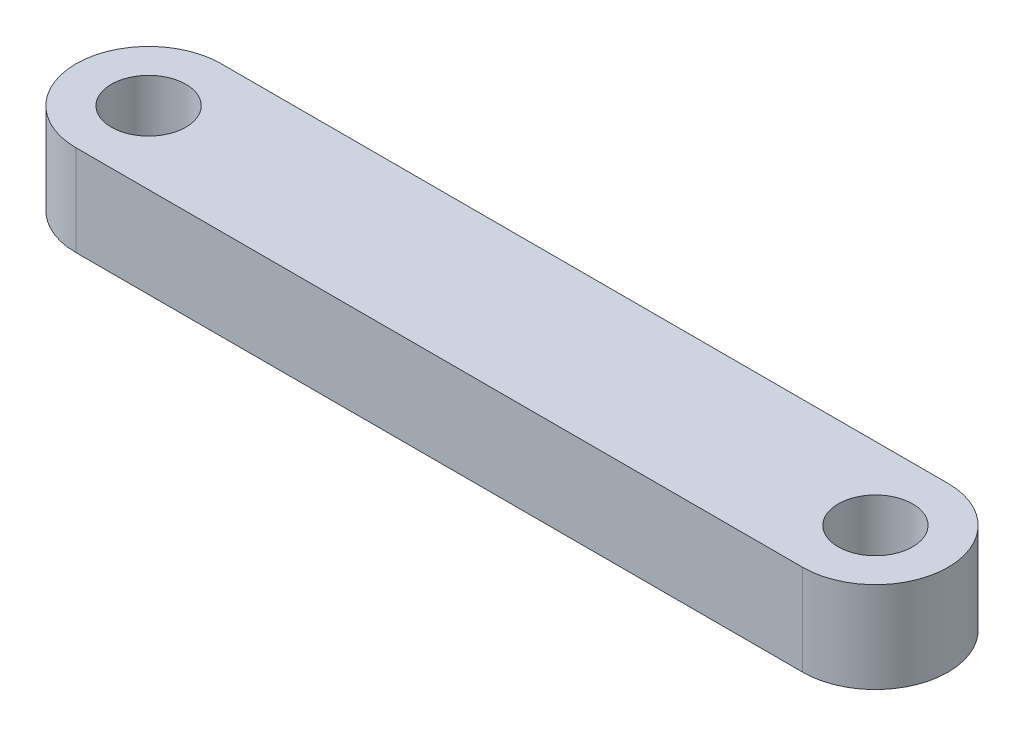
from build123d import *

# Parameters (mm, degrees)
SKETCH1_R           = 2.9
BOSS_EXTRUDE1_DEPTH = 6.35
BOSS_EXTRUDE2_START = -6.35
SKETCH2_R           = 2.9
SKETCH2_R_2         = 2.6035
BOSS_EXTRUDE2_DEPTH = 6.35


with BuildPart() as part:
    # Sketch1 → Boss-Extrude1 (new body)
    with BuildSketch(Plane(origin=(0, 0, 0), x_dir=(1, 0, 0), z_dir=(0, 1, 0))):
        with BuildLine():
            Line((0, 5.08), (50.8, 5.08))
            ThreePointArc((50.8, 5.08), (55.88, 0), (50.8, -5.08))
            Line((50.8, -5.08), (0, -5.08))
            ThreePointArc((0, -5.08), (-5.08, 0), (0, 5.08))
        make_face()
        with Locations(Location((0, 0, 0), (0, 0, 270))):
            Circle(SKETCH1_R, mode=Mode.SUBTRACT)
        with Locations(Location((50.8, 0, 0), (0, 0, 270))):
            Circle(SKETCH1_R, mode=Mode.SUBTRACT)
    extrude(amount=BOSS_EXTRUDE1_DEPTH)

    # Sketch2 → Boss-Extrude2 (add)
    # profile 1 of 2: a face of its own
    with BuildSketch(Plane(origin=(0, 6.35, 0), x_dir=(1, 0, 0), z_dir=(0, 1, 0)).offset(BOSS_EXTRUDE2_START)):
        Circle(SKETCH2_R)
        with Locations(Location((0, 0, 0), (0, 0, 270))):
            Circle(SKETCH2_R_2, mode=Mode.SUBTRACT)
    # profile 2 of 2: a face of its own
    with BuildSketch(Plane(origin=(0, 6.35, 0), x_dir=(1, 0, 0), z_dir=(0, 1, 0)).offset(BOSS_EXTRUDE2_START)):
        with Locations((50.8, 0)):
            Circle(SKETCH2_R)
        with Locations(Location((50.8, 0, 0), (0, 0, 270))):
            Circle(SKETCH2_R_2, mode=Mode.SUBTRACT)
    extrude(amount=BOSS_EXTRUDE2_DEPTH)


solid = part.part
